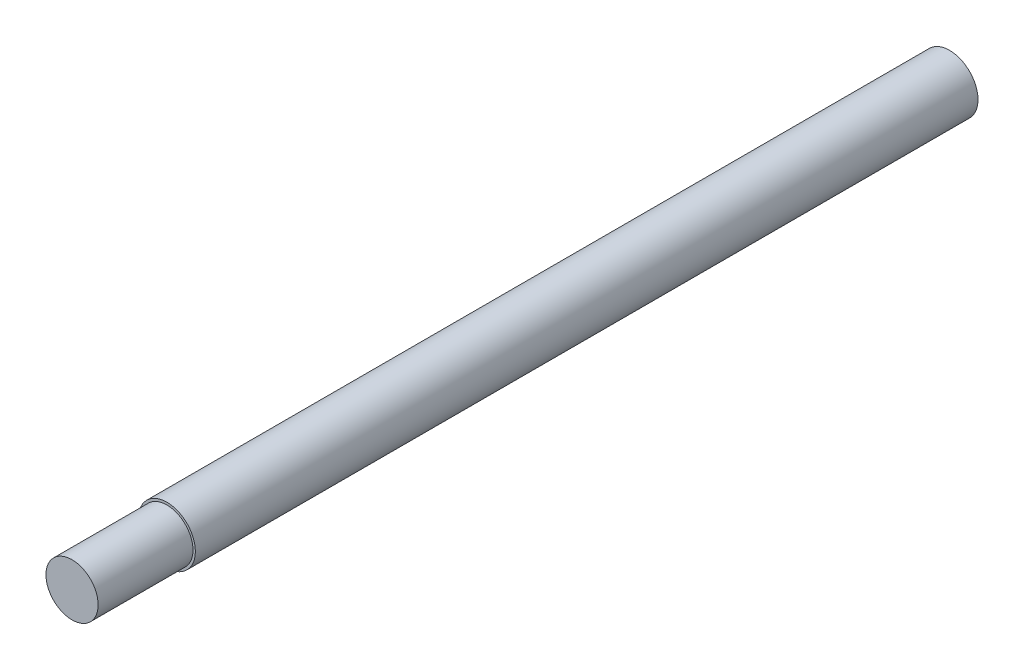
SolidWorks part; units mm, degrees
ref_plane "前视基准面" through (0, 0, 0) normal (0, 0, 1) x (1, 0, 0)
ref_plane "上视基准面" through (0, 0, 0) normal (0, 1, 0) x (1, 0, 0)
ref_plane "右视基准面" through (0, 0, 0) normal (1, 0, 0) x (0, 0, -1)
sketch "草图1" plane through (0, 0, 0) normal (0, 0, 1) x (1, 0, 0)
  circle A0 centre (0, 0) radius 6
  dimension "D1" = 12
extrude "凸台-拉伸3" add sketch "草图1" along normal mid plane 185
sketch "草图3" plane through (0, 0, 92.5) normal (0, 0, 1) x (1, 0, 0)
  circle A0 centre (0, 0) radius 5.5
  circle A1 centre (0, 0) radius 6 construction
  circle A2 centre (0, 0) radius 6
  dimension "D1" = 11
extrude "切除-拉伸1" cut sketch "草图3" against normal blind 20
cosmetic thread "装饰螺纹线1" parameters "D2"=10
